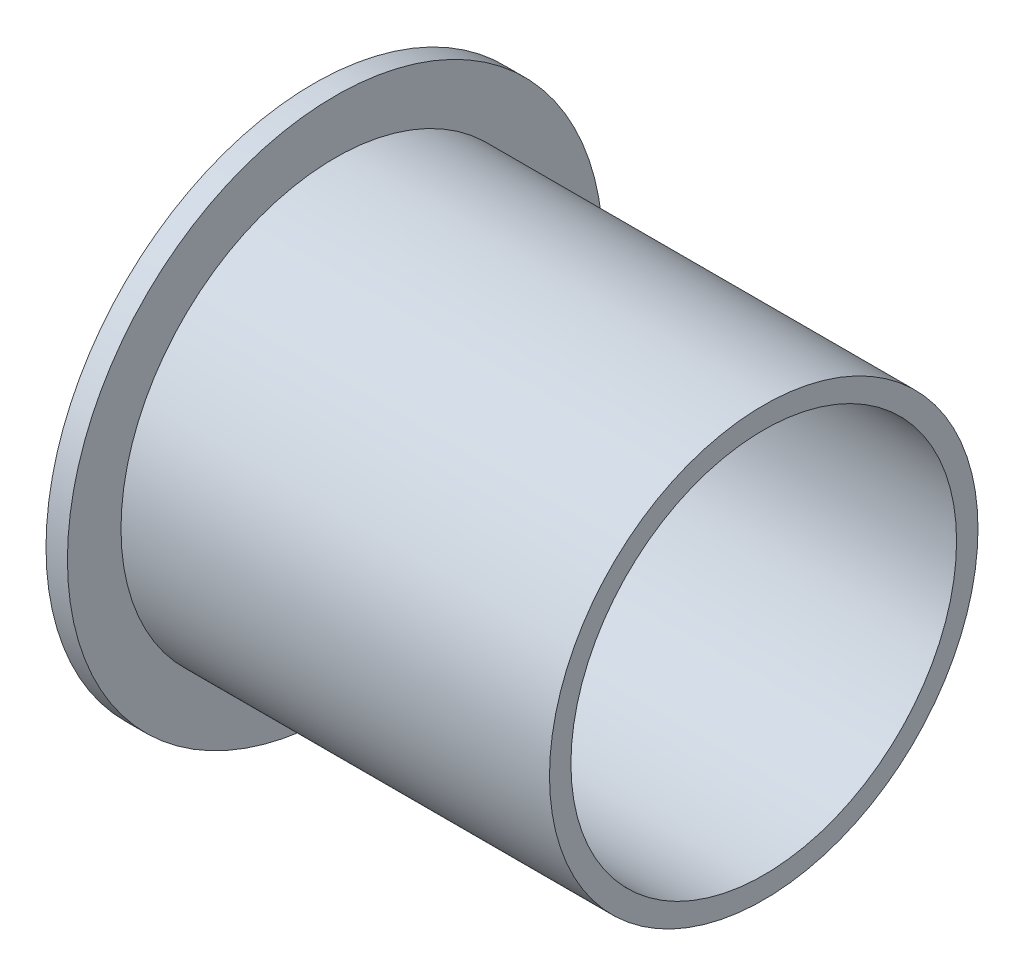
from build123d import *


with BuildPart() as part:
    # 草图1 → 旋转1 (revolve)
    with BuildSketch(Plane.XY, mode=Mode.PRIVATE) as revolve_1_sk:
        Polygon((0, 25), (2, 25), (2, 20), (42, 20), (42, 18), (2, 18), (2, 5), (0, 5), align=None)
    revolve(revolve_1_sk.sketch.rotate(Axis((0, 0, 0), (1, 0, 0)), 90), axis=Axis((0, 0, 0), (1, 0, 0)))


solid = part.part
